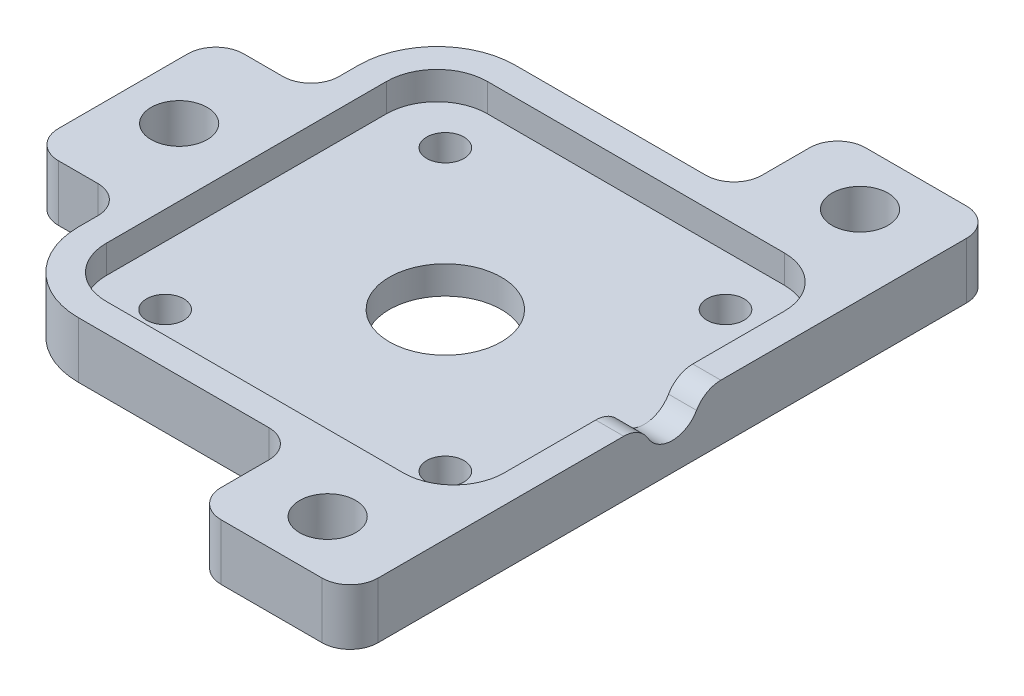
from build123d import *

# Parameters (mm, degrees)
SKETCH1_W           = 81
SKETCH1_H           = 78
SKETCH1_W_2         = 71
SKETCH1_H_2         = 68
BOSS_EXTRUDE1_DEPTH = 5
SKETCH2_W           = 81
SKETCH2_H           = 78
BOSS_EXTRUDE2_DEPTH = 5
BOSS_EXTRUDE3_DEPTH = 10
FILLET1_R           = 9
FILLET2_R           = 14
FILLET4_R           = 5
SKETCH4_R           = 10
CUT_EXTRUDE1_DEPTH  = 5
SKETCH5_R           = 5
CUT_EXTRUDE2_DEPTH  = 24
SKETCH6_R           = 5
CUT_EXTRUDE3_DEPTH  = 5
FILLET5_R           = 5
SKETCH7_R           = 3.3235
CUT_EXTRUDE4_DEPTH  = 10


with BuildPart() as part:
    # Sketch1 → Boss-Extrude1 (new body)
    with BuildSketch(Plane(origin=(0, 0, 0), x_dir=(1, 0, 0), z_dir=(0, 1, 0))):
        Rectangle(SKETCH1_W, SKETCH1_H)
        Rectangle(SKETCH1_W_2, SKETCH1_H_2, mode=Mode.SUBTRACT)
    extrude(amount=BOSS_EXTRUDE1_DEPTH)

    # Sketch2 → Boss-Extrude2 (add)
    with BuildSketch(Plane.XZ):
        Rectangle(SKETCH2_W, SKETCH2_H)
    extrude(amount=BOSS_EXTRUDE2_DEPTH)

    # Sketch3 → Boss-Extrude3 (add)
    with BuildSketch(Plane.XZ.offset(5)):
        Polygon((-42.5, 16.525991305), (-57.5, 16.525991305), (-57.5, 1.525991305), (-57.5, -1.525991305), (-57.5, -16.525991305), (-43.129437713, -16.525991305), (-40.5, -16.525991305), (-40.5, 16.525991305), align=None)
        Polygon((40.5, 57.5), (12.5, 57.5), (12.5, 42.5), (12.5, 39), (40.5, 39), align=None)
        Polygon((12.5, -39), (40.5, -39), (40.5, -57.5), (12.5, -57.5), (12.5, -42.5), align=None)
    extrude(amount=-BOSS_EXTRUDE3_DEPTH)

    # Fillet1
    fillet1_edges = [part.edges().sort_by_distance(p)[0] for p in [
        (35.5, 2.5, 34),
        (35.5, 2.5, -34),
        (-35.5, 2.5, -34),
        (-35.5, 2.5, 34),
    ]]
    fillet(fillet1_edges, radius=FILLET1_R)

    # Fillet2
    fillet2_edges = [part.edges().sort_by_distance(p)[0] for p in [
        (-40.5, 0, -39),
        (-40.5, 0, 39),
    ]]
    fillet(fillet2_edges, radius=FILLET2_R)

    # Fillet4
    fillet4_edges = [part.edges().sort_by_distance(p)[0] for p in [
        (-40.5, 0, 16.525991305),
        (-40.5, 0, -16.525991305),
        (-57.5, 0, -16.525991305),
        (-57.5, 0, 16.525991305),
        (12.5, 0, -39),
        (40.5, 0, -57.5),
        (12.5, 0, -57.5),
        (12.5, 0, 57.5),
        (40.5, 0, 57.5),
        (12.5, 0, 39),
    ]]
    fillet(fillet4_edges, radius=FILLET4_R)

    # Sketch4 → Cut-Extrude1 (cut)
    with BuildSketch(Plane(origin=(0, 0, 0), x_dir=(1, 0, 0), z_dir=(0, 1, 0))):
        with Locations(Location((0, 0, 0), (0, 0, 270))):
            Circle(SKETCH4_R)
    extrude(amount=-CUT_EXTRUDE1_DEPTH, mode=Mode.SUBTRACT)

    # Sketch5 → Cut-Extrude2 (cut)
    with BuildSketch(Plane(origin=(0, 5, 0), x_dir=(1, 0, 0), z_dir=(0, 1, 0))):
        with Locations(Location((26.5, 47.5, 0), (0, 0, 270))):
            Circle(SKETCH5_R)
        with Locations(Location((26.5, -47.5, 0), (0, 0, 270))):
            Circle(SKETCH5_R)
        with Locations(Location((-47.5, 0, 0), (0, 0, 270))):
            Circle(SKETCH5_R)
    extrude(amount=-CUT_EXTRUDE2_DEPTH, mode=Mode.SUBTRACT)

    # Sketch6 → Cut-Extrude3 (cut)
    with BuildSketch(Plane(origin=(40.5, 0, 0), x_dir=(0, 0, -1), z_dir=(1, 0, 0))):
        with Locations((0, 5)):
            Circle(SKETCH6_R)
    extrude(amount=-CUT_EXTRUDE3_DEPTH, mode=Mode.SUBTRACT)

    # Fillet5
    fillet5_edges = [part.edges().sort_by_distance(p)[0] for p in [
        (38, 5, 5),
        (38, 5, -5),
    ]]
    fillet(fillet5_edges, radius=FILLET5_R)

    # Sketch7 → Cut-Extrude4 (cut)
    with BuildSketch(Plane(origin=(0, 5, 0), x_dir=(1, 0, 0), z_dir=(0, 1, 0))):
        with Locations(Location((25, 25, 0), (0, 0, 270))):
            Circle(SKETCH7_R)
        with Locations(Location((-25, 25, 0), (0, 0, 270))):
            Circle(SKETCH7_R)
        with Locations(Location((-25, -25, 0), (0, 0, 270))):
            Circle(SKETCH7_R)
        with Locations(Location((25, -25, 0), (0, 0, 270))):
            Circle(SKETCH7_R)
    extrude(amount=-CUT_EXTRUDE4_DEPTH, mode=Mode.SUBTRACT)


solid = part.part
